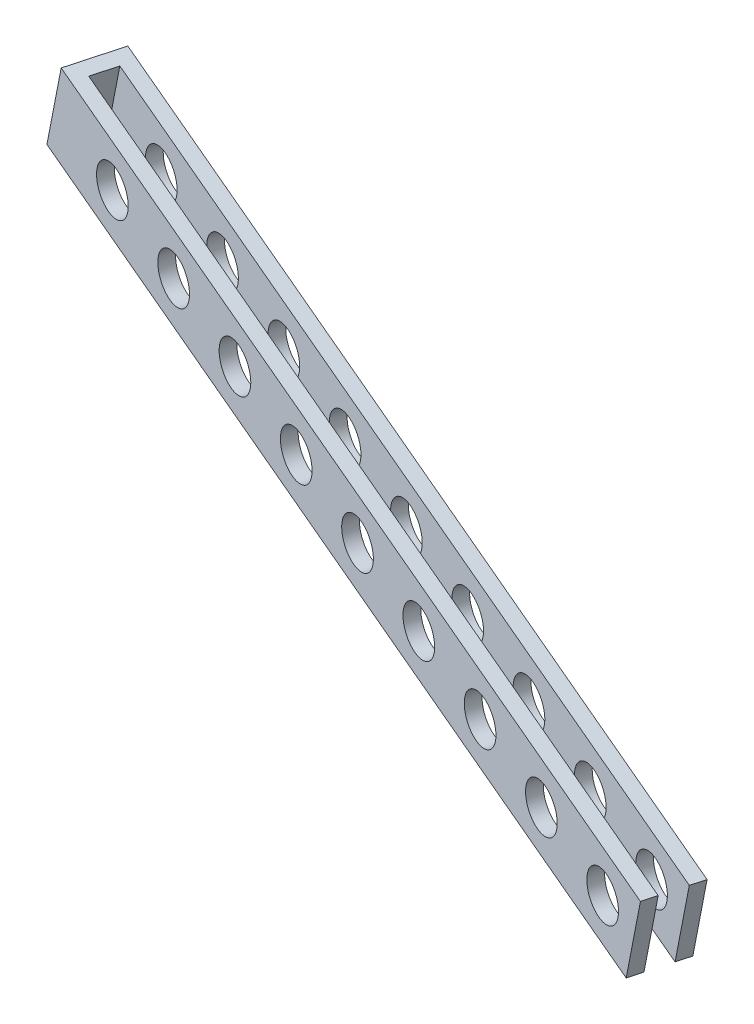
from build123d import *

# Parameters (mm, degrees)
EXTRUDE_THIN1_DEPTH      = 15
EXTRUDE_THIN1_DEPTH_BACK = 15
SKETCH2_R                = 12.5
CUT_EXTRUDE1_DEPTH       = 52
CUT_EXTRUDE2_DEPTH       = 52


with BuildPart() as part:
    # Sketch1 → Extrude-Thin1 (new, two sides: drawn at the far end of the back side and taken through both)
    with BuildSketch(Plane(origin=(-52.015152818, 0, 189.77373053), x_dir=(0.9644293353148398, 0, 0.2643407974266862), z_dir=(-0.2643407974266862, 0, 0.9644293353148398)).offset(-EXTRUDE_THIN1_DEPTH_BACK)):
        Polygon((-6.089055059, 159.279680039), (25.645783745, 151.090927797), (451.524648913, 41.198562071), (462.768022338, 84.771335153), (36.889157171, 194.663700878), (5.154318366, 202.85245312), align=None)
    extrude(amount=EXTRUDE_THIN1_DEPTH + EXTRUDE_THIN1_DEPTH_BACK)

    # Sketch2 → Cut-Extrude1 (cut)
    with BuildSketch(Plane(origin=(-55.98026478, 0, 204.240170559), x_dir=(0.9644293353148398, 0, 0.26434079742668615), z_dir=(-0.26434079742668615, 0, 0.9644293353148398))):
        with Locations((432.939239469, 69.231267182)):
            Circle(SKETCH2_R)
        with Locations((384.525047156, 81.723904321)):
            Circle(SKETCH2_R)
        with Locations((336.110854844, 94.216541461)):
            Circle(SKETCH2_R)
        with Locations((287.696662531, 106.7091786)):
            Circle(SKETCH2_R)
        with Locations((239.282470218, 119.20181574)):
            Circle(SKETCH2_R)
        with Locations((190.868277905, 131.694452879)):
            Circle(SKETCH2_R)
        with Locations((142.454085592, 144.187090019)):
            Circle(SKETCH2_R)
        with Locations((94.03989328, 156.679727158)):
            Circle(SKETCH2_R)
        with Locations((45.625700967, 169.172364298)):
            Circle(SKETCH2_R)
    extrude(amount=-CUT_EXTRUDE1_DEPTH, mode=Mode.SUBTRACT)

    # Sketch3 → Cut-Extrude2 (cut)
    with BuildSketch(Plane(origin=(47.64042684, 191.43608201, 13.057782421), x_dir=(0.9705337279727567, -0.24040671124001461, -0.01639805043483442), z_dir=(0.24096531465607895, 0.9682838462558588, 0.06604627326849857))):
        Polygon((359.082690346, -298.87451483), (355.26956046, -312.345225296), (-91.768329186, -185.803010492), (-87.955199299, -172.332300026), align=None)
    extrude(amount=-CUT_EXTRUDE2_DEPTH, mode=Mode.SUBTRACT)


solid = part.part
